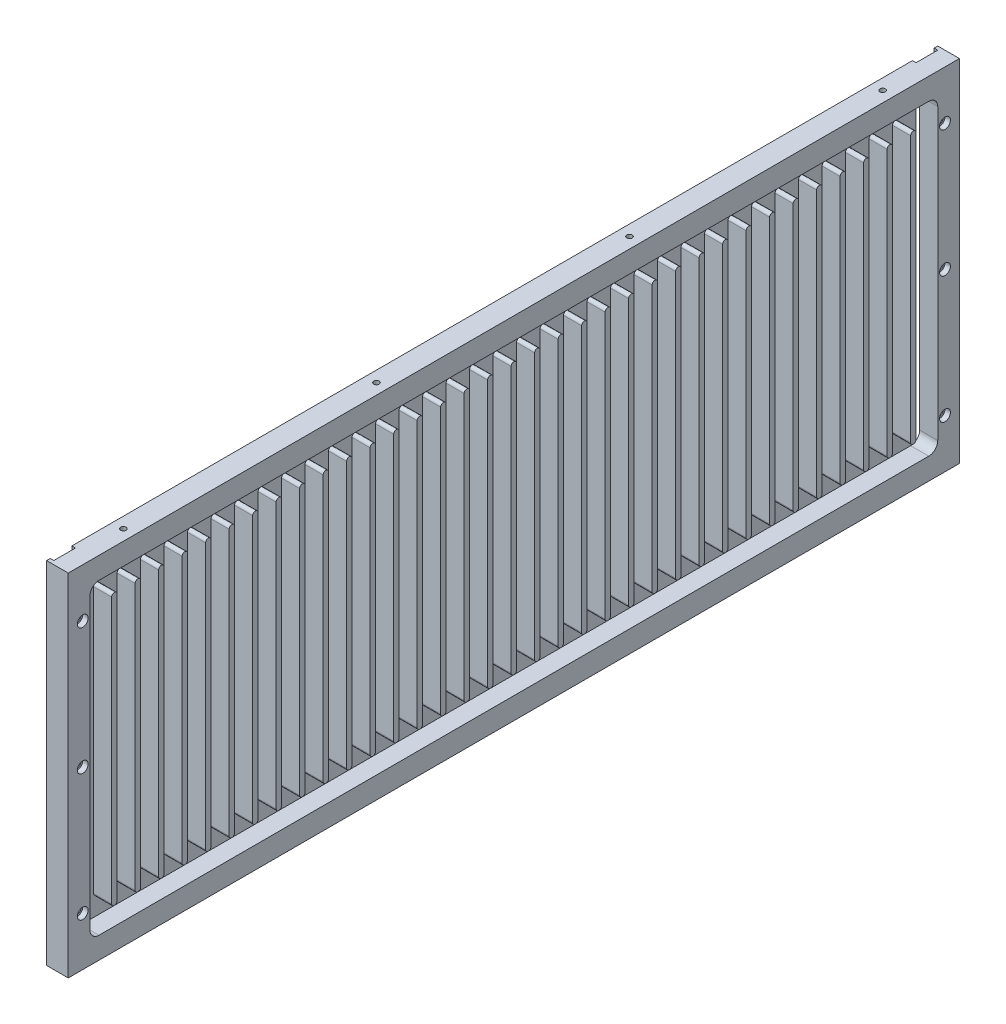
SolidWorks part; units mm, degrees
ref_plane "Front Plane" through (0, 0, 0) normal (0, 0, 1) x (1, 0, 0)
ref_plane "Top Plane" through (0, 0, 0) normal (0, 1, 0) x (1, 0, 0)
ref_plane "Right Plane" through (0, 0, 0) normal (1, 0, 0) x (0, 0, -1)
sketch "Sketch1" plane through (0, 0, 0) normal (1, 0, 0) x (0, 0, -1)
  line L1 (-246.5, 97) -> (246.5, 97)
  line L2 (-246.5, 97) -> (-246.5, -97)
  line L3 (-246.5, -97) -> (246.5, -97)
  line L4 (246.5, 97) -> (246.5, -97)
  line L5 (-246.5, 97) -> (246.5, -97) construction
  line L6 (-246.5, -97) -> (246.5, 97) construction
  point P0 (0, 0)
  dimension "D1" = 194
  dimension "D2" = 493
extrude "Boss-Extrude1" add sketch "Sketch1" along normal mid plane 12
sketch "Sketch2" plane through (6, 0, 0) normal (1, 0, 0) x (0, 0, -1)
  line L8 (234.5, -85) -> (234.5, 85)
  line L9 (234.5, 85) -> (-234.5, 85)
  line L10 (-234.5, 85) -> (-234.5, -85)
  line L11 (-234.5, -85) -> (234.5, -85)
  line L12 (234.5, -85) -> (234.5, 85)
  line L13 (234.5, 85) -> (-234.5, 85)
  line L14 (-234.5, 85) -> (-234.5, -85)
  line L15 (-234.5, -85) -> (234.5, -85)
  dimension "D1" = 12
extrude "Cut-Extrude1" cut sketch "Sketch2" against normal blind 10
sketch "Sketch3" plane through (-4, 0, 0) normal (1, 0, 0) x (0, 0, -1)
  line L0 (-1.9827, 0) -> (2.0505, 0) construction
  line L1 (-0.5, 75) -> (0.5, 75) construction
  line L2 (-1.5, 73.5) -> (-1.5, -73.5)
  line L3 (-0.5, -75) -> (0.5, -75) construction
  line L4 (1.5, 73.5) -> (1.5, -73.5)
  line L5 (-1.5, 75) -> (1.5, -75) construction
  line L6 (-1.5, -75) -> (1.5, 75) construction
  arc A0 (-1.5, 74) -> (-0.5, 75) centre (-0.5, 74) cw construction
  arc A1 (1.5, 74) -> (0.5, 75) centre (0.5, 74) ccw construction
  arc A2 (0.5, -75) -> (1.5, -74) centre (0.5, -74) ccw construction
  arc A3 (-1.5, -74) -> (-0.5, -75) centre (-0.5, -74) ccw construction
  arc A4 (1.5, 73.5) -> (-1.5, 73.5) centre (0, 73.5) ccw
  arc A5 (1.5, -73.5) -> (-1.5, -73.5) centre (0, -73.5) cw
  point P0 (0, 0)
  dimension "D3" = 1
  dimension "D4" = 1
  dimension "D5" = 1
  dimension "D6" = 3
  dimension "D1" = 3
  dimension "D2" = 150
extrude "Boss-Extrude2" add sketch "Sketch3" along normal blind 10
pattern_linear "LPattern1" count 18 spacing 13 along (0, 0, -1) count 18 spacing 13 along (0, 0, 1) seed only of "Boss-Extrude2"
fillet "Fillet1" radius 5 4 edges at (1, 85, 234.5) (1, -85, 234.5) (1, 85, -234.5) (1, -85, -234.5)
sketch "Sketch4" plane through (6, 0, 0) normal (1, 0, 0) x (0, 0, -1)
  line L0 (-293.2598, 0) -> (261.2548, 0) construction
  line L1 (-246.5, 97) -> (-246.5, -97) construction
  circle A0 centre (-238.5, 0) radius 2
  circle A1 centre (-238.5, 70) radius 2
  circle A2 centre (-238.5, -70) radius 2
  dimension "D1" = 4
  dimension "D2" = 8
  dimension "D3" = 4
  dimension "D4" = 70
extrude "Cut-Extrude2" cut sketch "Sketch4" against normal through all
mirror "Mirror1" about plane through (0, 0, 0) normal (0, 0, 1) of "Cut-Extrude2"
sketch "Sketch5" plane through (-6, 0, 0) normal (-1, 0, 0) x (0, 0, 1)
  line L0 (238.5, 134.2014) -> (238.5, -136.3189) construction
  line L1 (-246.5, 97) -> (246.5, 97) construction
  line L2 (244.5, -97) -> (232.5, -97)
  line L3 (244.5, -97) -> (244.5, 97)
  line L4 (244.5, 97) -> (232.5, 97)
  line L5 (232.5, -97) -> (232.5, 97)
  line L6 (244.5, -97) -> (232.5, 97) construction
  line L7 (244.5, 97) -> (232.5, -97) construction
  point P3 (238.5, 0)
  dimension "D1" = 12
extrude "Cut-Extrude3" cut sketch "Sketch5" against normal blind 2
mirror "Mirror2" about plane through (0, 0, 0) normal (0, 0, 1) of "Cut-Extrude3"
sketch "Sketch6" plane through (0, 97, 0) normal (0, 1, 0) x (1, 0, 0)
  line L0 (-33.7051, 0) -> (45.266, 0) construction
  line L1 (0, 268.9466) -> (0, -293.5781) construction
  circle A0 centre (0, -70) radius 1.5
  circle A1 centre (0, -210) radius 1.5
  circle A2 centre (0, 210) radius 1.5
  circle A3 centre (0, 70) radius 1.5
  dimension "D1" = 3
  dimension "D2" = 3
  dimension "D3" = 70
  dimension "D4" = 140
extrude "Cut-Extrude4" cut sketch "Sketch6" against normal blind 4
mirror "Mirror3" about plane through (0, 0, 0) normal (0, 1, 0) of "Cut-Extrude4"
sketch "Sketch7" plane through (6, 0, 0) normal (1, 0, 0) x (0, 0, -1)
  circle A0 centre (238.5, 0) radius 3
  circle A1 centre (238.5, 70) radius 3
  circle A2 centre (238.5, -70) radius 3
  circle A3 centre (-238.5, -70) radius 3
  circle A4 centre (-238.5, 0) radius 3
  circle A6 centre (-238.5, 70) radius 3
  dimension "D1" = 6
extrude "Cut-Extrude5" cut sketch "Sketch7" against normal blind 3
